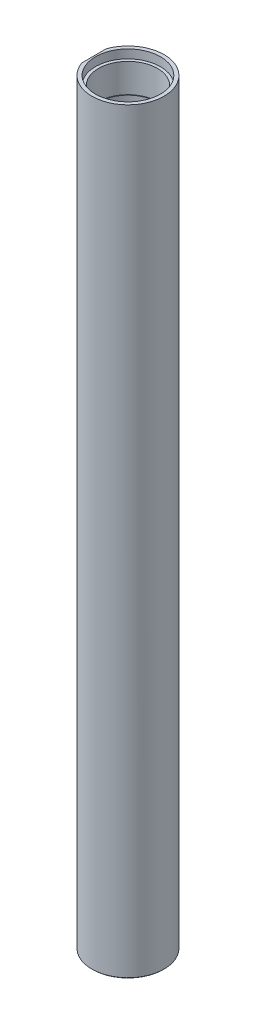
SolidWorks part; units mm, degrees
material "AISI 1045 钢，冷拔"
ref_plane "Front Plane" through (0, 0, 0) normal (0, 0, 1) x (1, 0, 0)
ref_plane "Top Plane" through (0, 0, 0) normal (0, 1, 0) x (1, 0, 0)
ref_plane "Right Plane" through (0, 0, 0) normal (1, 0, 0) x (0, 0, -1)
sketch "Sketch1" plane through (0, 0, 0) normal (0, 1, 0) x (1, 0, 0)
  circle A0 centre (0, 0) radius 40
  circle A1 centre (0, 0) radius 50
  dimension "D1" = 80
  dimension "D2" = 100
extrude "Boss-Extrude1" add sketch "Sketch1" along normal blind 1049
sketch "Sketch10" plane through (0, 1049, 0) normal (0, 1, 0) x (1, 0, 0)
  circle A0 centre (0, 0) radius 45
  dimension "D1" = 90
extrude "Cut-Extrude8" cut sketch "Sketch10" against normal blind 12
sketch "Sketch13" plane through (0, 0, 0) normal (0, -1, 0) x (1, 0, 0)
  circle A0 centre (0, 0) radius 44.375
  dimension "D1" = 88.75
extrude "Cut-Extrude10" cut sketch "Sketch13" against normal blind 40
cosmetic thread "Cosmetic Thread3" parameters "D1"=35, "D2"=92
chamfer "Chamfer5" distance 1 angle 45 2 edges at (0, 0, 50) (0, 0, -44.375)
sketch "Sketch14" plane through (0, 1037, 0) normal (0, 1, 0) x (1, 0, 0)
  circle A0 centre (0, 0) radius 40.875
  dimension "D1" = 81.75
extrude "Cut-Extrude11" cut sketch "Sketch14" against normal blind 40
cosmetic thread "Cosmetic Thread2" parameters "D1"=35, "D2"=85
sketch "Sketch15" plane through (0, 0, 0) normal (0, 0, 1) x (1, 0, 0)
  line L0 (50, 1049) -> (-50, 1049) construction
  line L1 (-53, 1069) -> (-47, 1069)
  line L2 (-53, 1069) -> (-53, 1029)
  line L3 (-53, 1029) -> (-47, 1029)
  line L4 (-47, 1069) -> (-47, 1029)
  line L5 (-53, 1069) -> (-47, 1029) construction
  line L6 (-53, 1029) -> (-47, 1069) construction
  point P0 (-50, 1049)
  dimension "D1" = 20
  dimension "D2" = 6
extrude "Cut-Extrude12" cut sketch "Sketch15" against normal through all both and the other way through all
